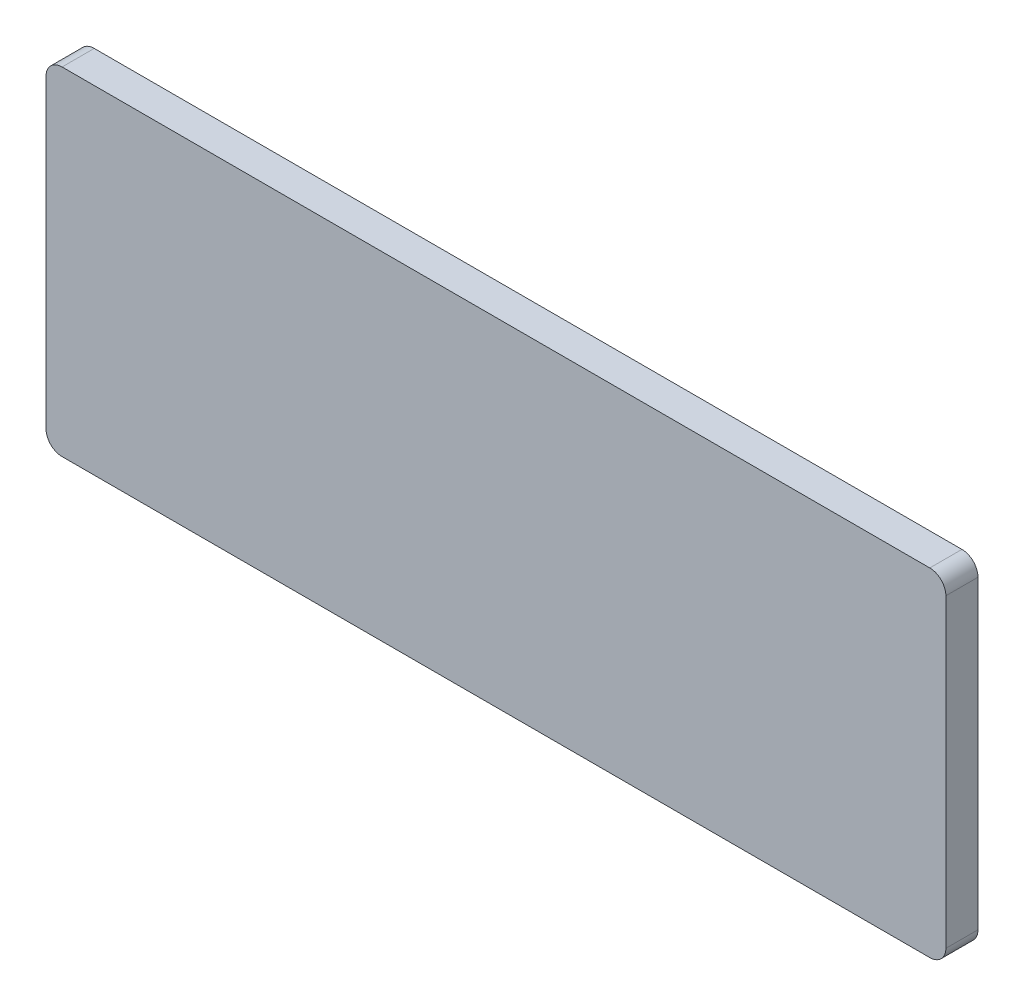
SolidWorks part; units mm, degrees
material "1023 Carbon Steel Plate (SS)"
ref_plane "Front Plane" through (0, 0, 0) normal (0, 0, 1) x (1, 0, 0)
ref_plane "Top Plane" through (0, 0, 0) normal (0, 1, 0) x (1, 0, 0)
ref_plane "Right Plane" through (0, 0, 0) normal (1, 0, 0) x (0, 0, -1)
sketch "Sketch1" plane through (0, 0, 0) normal (0, 0, 1) x (1, 0, 0)
  line L1 (54, 21) -> (-54, 21)
  line L2 (56, 19) -> (56, -19)
  line L3 (54, -21) -> (-54, -21)
  line L4 (-56, 19) -> (-56, -19)
  line L5 (56, 21) -> (-56, -21) construction
  line L6 (56, -21) -> (-56, 21) construction
  arc A0 (-54, -21) -> (-56, -19) centre (-54, -19) cw
  arc A1 (56, -19) -> (54, -21) centre (54, -19) cw
  arc A2 (54, 21) -> (56, 19) centre (54, 19) cw
  arc A3 (-54, 21) -> (-56, 19) centre (-54, 19) ccw
  point P0 (0, 0)
  dimension "D3" = 2
  dimension "D1" = 112
  dimension "D2" = 42
extrude "Boss-Extrude1" add sketch "Sketch1" along normal blind 4 contours L4 A0 L3 A1 L2 A2 L1 A3
